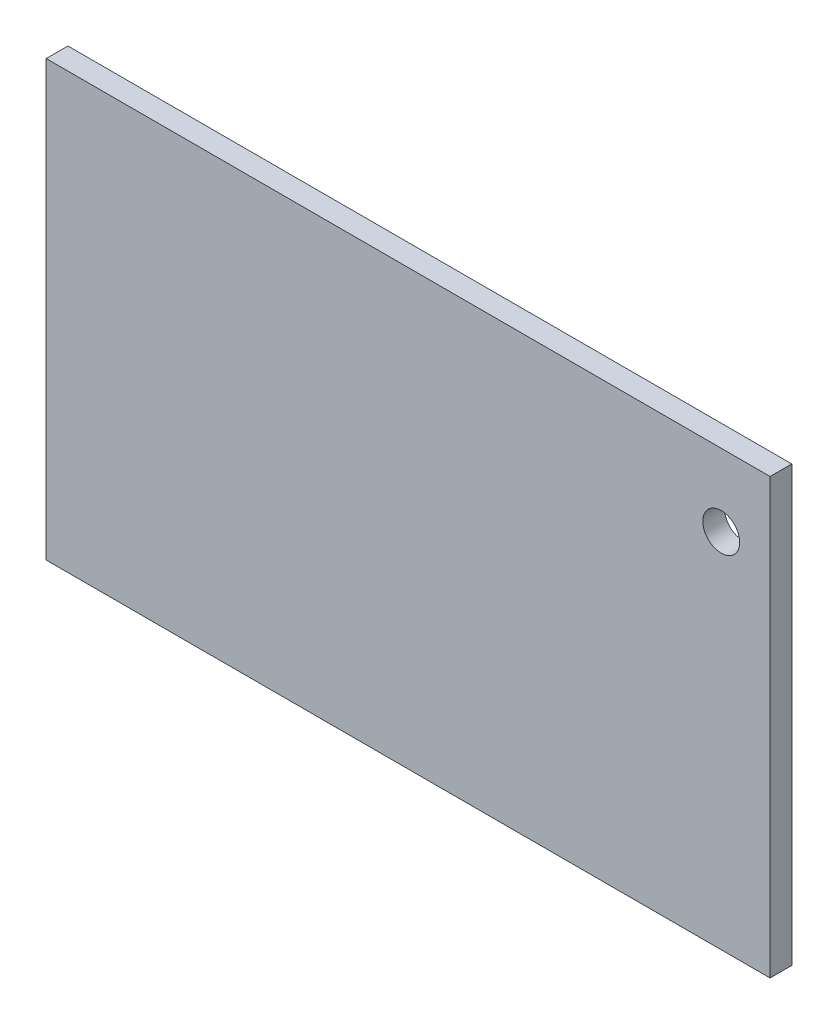
from build123d import *

# Parameters (mm, degrees)
SKETCH1_W              = 200
SKETCH1_H              = 120
BOSS_EXTRUDE1_DEPTH    = 6
M12_TAPPED_HOLE1_D     = 10.2
M12_TAPPED_HOLE1_DEPTH = 29.25
M12_TAPPED_HOLE1_TIP   = 3.064389157


with BuildPart() as part:
    # Sketch1 → Boss-Extrude1 (new body)
    with BuildSketch(Plane.XY):
        Rectangle(SKETCH1_W, SKETCH1_H)
    extrude(amount=BOSS_EXTRUDE1_DEPTH)

    # M12 Tapped Hole1
    with Locations(Plane.XY.offset(6)):
        with Locations((86.5, 40)):
            Hole(M12_TAPPED_HOLE1_D / 2, depth=M12_TAPPED_HOLE1_DEPTH)
            with Locations((0, 0, -(M12_TAPPED_HOLE1_DEPTH + M12_TAPPED_HOLE1_TIP / 2))):  # 118° drill point
                Cone(0, M12_TAPPED_HOLE1_D / 2, M12_TAPPED_HOLE1_TIP, mode=Mode.SUBTRACT)


solid = part.part
